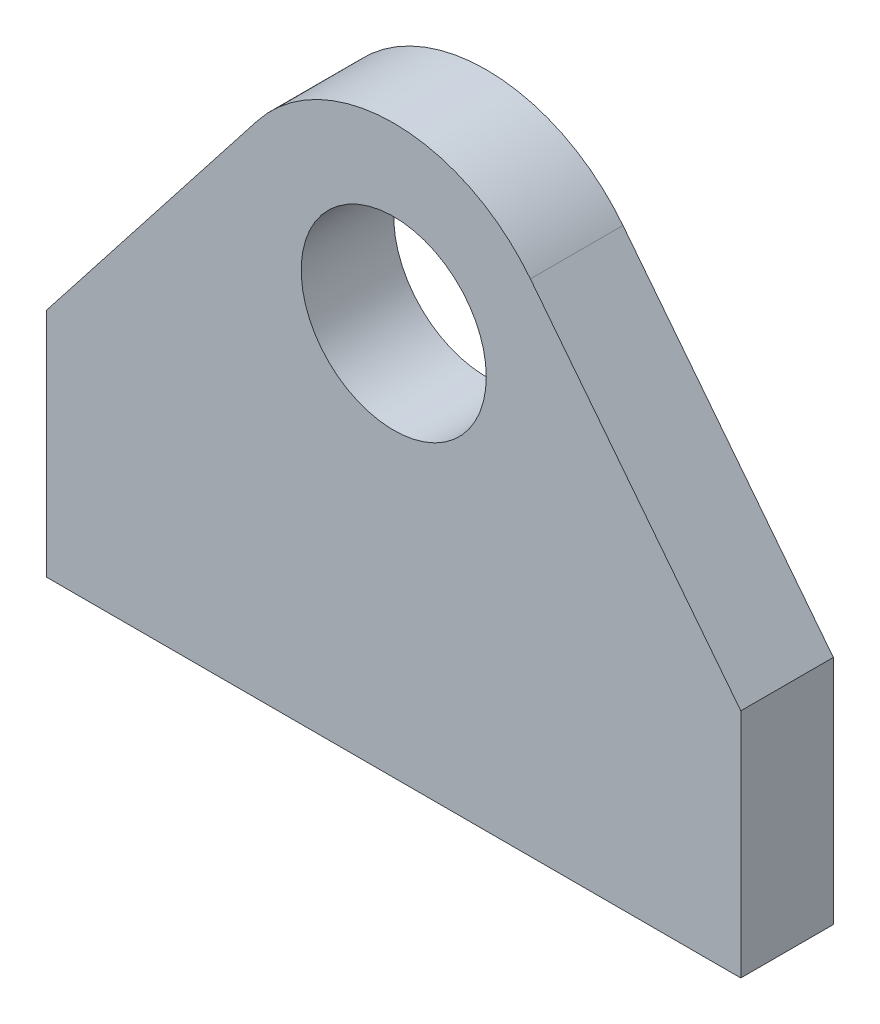
SolidWorks part; units mm, degrees
material "普通碳钢"
ref_plane "Front Plane" through (0, 0, 0) normal (0, 0, 1) x (1, 0, 0)
ref_plane "Top Plane" through (0, 0, 0) normal (0, 1, 0) x (1, 0, 0)
ref_plane "Right Plane" through (0, 0, 0) normal (1, 0, 0) x (0, 0, -1)
sketch "Sketch1" plane through (0, 0, 0) normal (0, 0, 1) x (1, 0, 0)
  line L0 (0, 0) -> (0, 20)
  line L1 (0, 0) -> (60, 0)
  line L2 (60, 0) -> (60, 20)
  line L3 (60, 20) -> (41.8136, 43.2434)
  line L4 (0, 20) -> (18.1864, 43.2434)
  line L5 (30, 34) -> (30, 0) construction
  arc A0 (41.8136, 43.2434) -> (18.1864, 43.2434) centre (30, 34) ccw
  circle A1 centre (30, 34) radius 8
  dimension "D4" = 30
  dimension "D5" = 16
  dimension "D1" = 20
  dimension "D2" = 34
  dimension "D3" = 60
extrude "Boss-Extrude1" add sketch "Sketch1" along normal blind 8
